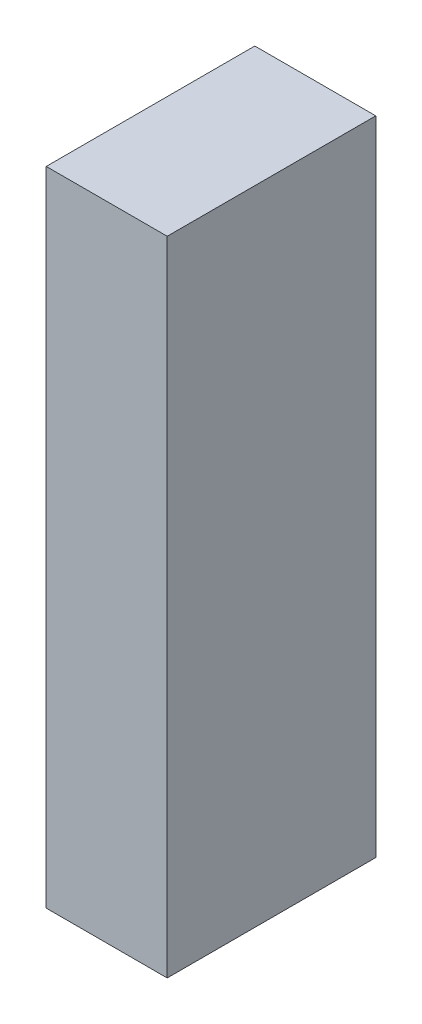
SolidWorks part; units mm, degrees
material "Q235A"
ref_plane "Front Plane" through (0, 0, 0) normal (0, 0, 1) x (1, 0, 0)
ref_plane "Top Plane" through (0, 0, 0) normal (0, 1, 0) x (1, 0, 0)
ref_plane "Right Plane" through (0, 0, 0) normal (1, 0, 0) x (0, 0, -1)
sketch "Sketch1" plane through (0, 0, 0) normal (0, 0, 1) x (1, 0, 0)
  line L1 (7.25, -38.5) -> (-7.25, -38.5)
  line L2 (7.25, -38.5) -> (7.25, 38.5)
  line L3 (7.25, 38.5) -> (-7.25, 38.5)
  line L4 (-7.25, -38.5) -> (-7.25, 38.5)
  line L5 (7.25, -38.5) -> (-7.25, 38.5) construction
  line L6 (7.25, 38.5) -> (-7.25, -38.5) construction
  point P0 (0, 0)
  dimension "D1" = 14.5
  dimension "D2" = 77
extrude "Boss-Extrude1" add sketch "Sketch1" along normal blind 25
